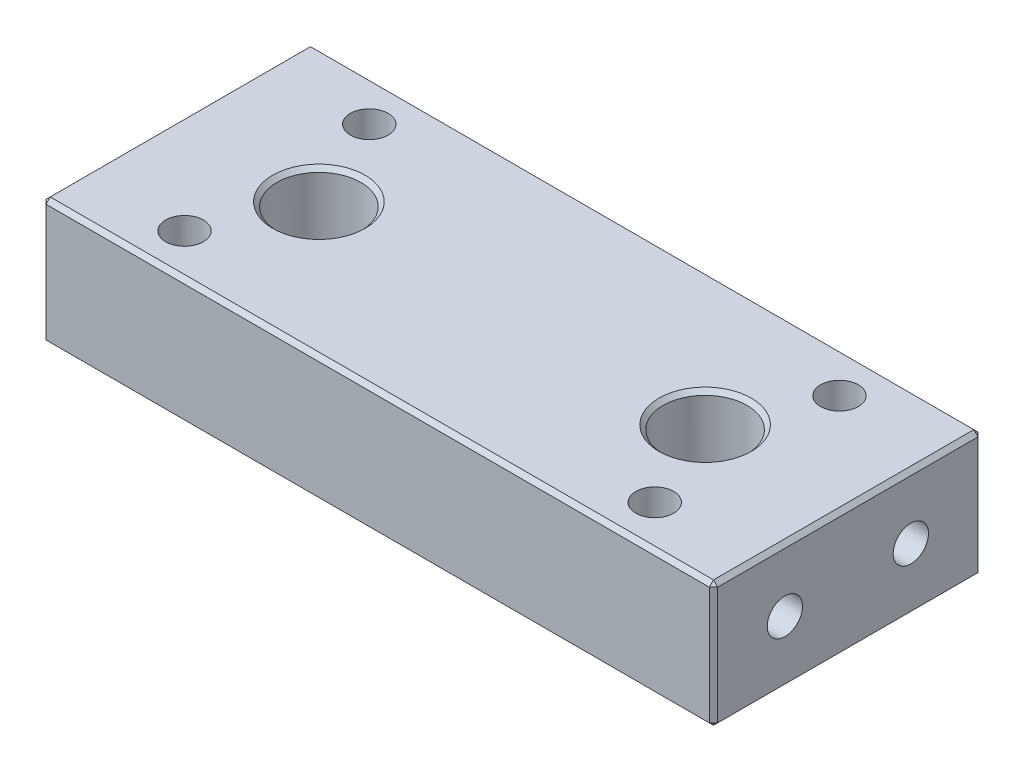
SolidWorks part; units mm, degrees
material "A7075"
ref_plane "Front Plane" through (0, 0, 0) normal (0, 0, 1) x (1, 0, 0)
ref_plane "Top Plane" through (0, 0, 0) normal (0, 1, 0) x (1, 0, 0)
ref_plane "Right Plane" through (0, 0, 0) normal (1, 0, 0) x (0, 0, -1)
sketch "Sketch1" plane through (0, 0, 0) normal (0, 0, 1) x (1, 0, 0)
  line L1 (0, 0) -> (80, 0)
  line L3 (40, 0) -> (40, -51.8024) construction
  dimension "D1" = 80
extrude "Extrude-Thin1" add sketch "Sketch1" along normal mid plane 32 thin
hole_wizard "Hole size by socket head cap screw type1" positions "Sketch3" profile "Sketch2" counterbore size "M4" standard "Gb" end condition through all
sketch "Sketch3" plane through (0, -15, 0) normal (0, -1, 0) x (-1, 0, 0)
  line L1 (-12, -11) -> (-68, -11) construction
  line L2 (-12, -11) -> (-12, 11) construction
  line L3 (-12, 11) -> (-68, 11) construction
  line L4 (-68, -11) -> (-68, 11) construction
  line L7 (0, 0) -> (-67.9842, 0) construction
  line L8 (-40, 16) -> (-40, -32.9152) construction
  line L11 (0, 16) -> (-80, 16) construction
  point P0 (-68, -11)
  point P2 (-68, 11)
  point P4 (-12, -11)
  point P6 (-12, 11)
  dimension "D2" = 22
  dimension "D3" = 56
sketch "Sketch2" plane through (68, -15, 11) normal (1, 0, 0) x (0, 0, -1)
  line L0 (0, 0) -> (0, 15)
  line L1 (0, 15) -> (2.25, 15)
  line L3 (2.25, 15) -> (2.25, 4.6)
  line L4 (2.25, 4.6) -> (4, 4.6)
  line L5 (4, 4.6) -> (4, 0)
  line L7 (4, 0) -> (0, 0)
  line L11 (0, -6.35) -> (0, 107.95) construction
  dimension "通孔孔直径" = 4.5
  dimension "通孔孔深度" = 15
  dimension "柱形沉头孔直径" = 8
  dimension "柱形沉头孔深度" = 4.6
sketch "Sketch4" plane through (0, -15, 0) normal (0, -1, 0) x (1, 0, 0)
  line L0 (12, 11) -> (68, 11) construction
  line L1 (40, 11) -> (40, -12.5314) construction
  circle A0 centre (17, 0) radius 5
  circle A1 centre (63, 0) radius 5
  dimension "D1" = 46
  dimension "D2" = 10
extrude "Cut-Extrude1" cut sketch "Sketch4" against normal through all
hole_wizard "M5 Tapped Hole2" positions "Sketch6" profile "Sketch5" tap size "M5" standard "Gb"
sketch "Sketch6" plane through (80, 0, 0) normal (1, 0, 0) x (0, 0, -1)
  line L5 (0, 28.5562) -> (0, -30.7287) construction
  line L9 (16, -7.5) -> (-16, -7.5) construction
  line L10 (16, 0) -> (16, -15) construction
  line L11 (-16, 0) -> (-16, -15) construction
  point P0 (-7.5, -7.5)
  point P2 (7.5, -7.5)
  dimension "D1" = 15
sketch "Sketch5" plane through (80, -7.5, 7.5) normal (0, 1, 0) x (0, 0, -1)
  line L0 (0, 0) -> (0, 11.2618)
  line L1 (0, 11.2618) -> (2.1, 10)
  line L2 (2.1, 10) -> (2.1, 0)
  line L5 (2.1, 0) -> (0, 0)
  line L10 (0, 11.2618) -> (-2.1, 10) construction
  line L11 (0, -6.35) -> (0, 107.95) construction
  dimension "螺纹孔钻头直径" = 4.2
  dimension "螺纹孔钻头深度" = 10
  dimension "导头角度" = 118
cosmetic thread "Cosmetic Thread1" parameters "D1"=10, "D2"=5
cosmetic thread "Cosmetic Thread2" parameters "D1"=10, "D2"=5
hole_wizard "M5 Tapped Hole1" positions "Sketch8" profile "Sketch10" tap size "M5" standard "Gb"
sketch "Sketch8" plane through (0, -24.3152, 11.7091) normal (-1, 0, 0) x (0, 0, 1)
  line L5 (-11.7091, 28.5562) -> (-11.7091, 9.3152) construction
  line L9 (4.2909, 16.8152) -> (-27.7091, 16.8152) construction
  line L10 (4.2909, 9.3152) -> (4.2909, 24.3152) construction
  line L11 (-27.7091, 9.3152) -> (-27.7091, 24.3152) construction
  line L12 (4.2909, 9.3152) -> (-27.7091, 9.3152) construction
  point P0 (-19.2091, 16.8152)
  point P2 (-4.2091, 16.8152)
  dimension "D1" = 15
sketch "Sketch10" plane through (0, -7.5, -7.5) normal (0, 1, 0) x (0, 0, 1)
  line L0 (0, 0) -> (0, 11.2618)
  line L1 (0, 11.2618) -> (2.1, 10)
  line L2 (2.1, 10) -> (2.1, 0)
  line L5 (2.1, 0) -> (0, 0)
  line L10 (0, 11.2618) -> (-2.1, 10) construction
  line L11 (0, -6.35) -> (0, 107.95) construction
  dimension "螺纹孔钻头直径" = 4.2
  dimension "螺纹孔钻头深度" = 10
  dimension "导头角度" = 118
cosmetic thread "Cosmetic Thread4" parameters "D1"=10, "D2"=5
cosmetic thread "Cosmetic Thread5" parameters "D1"=10, "D2"=5
chamfer "Chamfer1" distance 0.5 angle 45 16 edges at (40, -15, 16) (80, -15, 0) (40, -15, -16) (40, 0, 16) (80, 0, 0) (40, 0, -16) (80, -7.5, -16) (80, -7.5, 16) (0, -7.5, 16) (0, -7.5, -16) (63, 0, -5) (63, -15, -5) (17, 0, -5) (17, -15, -5) (0, -15, 0) (0, 0, 0)
